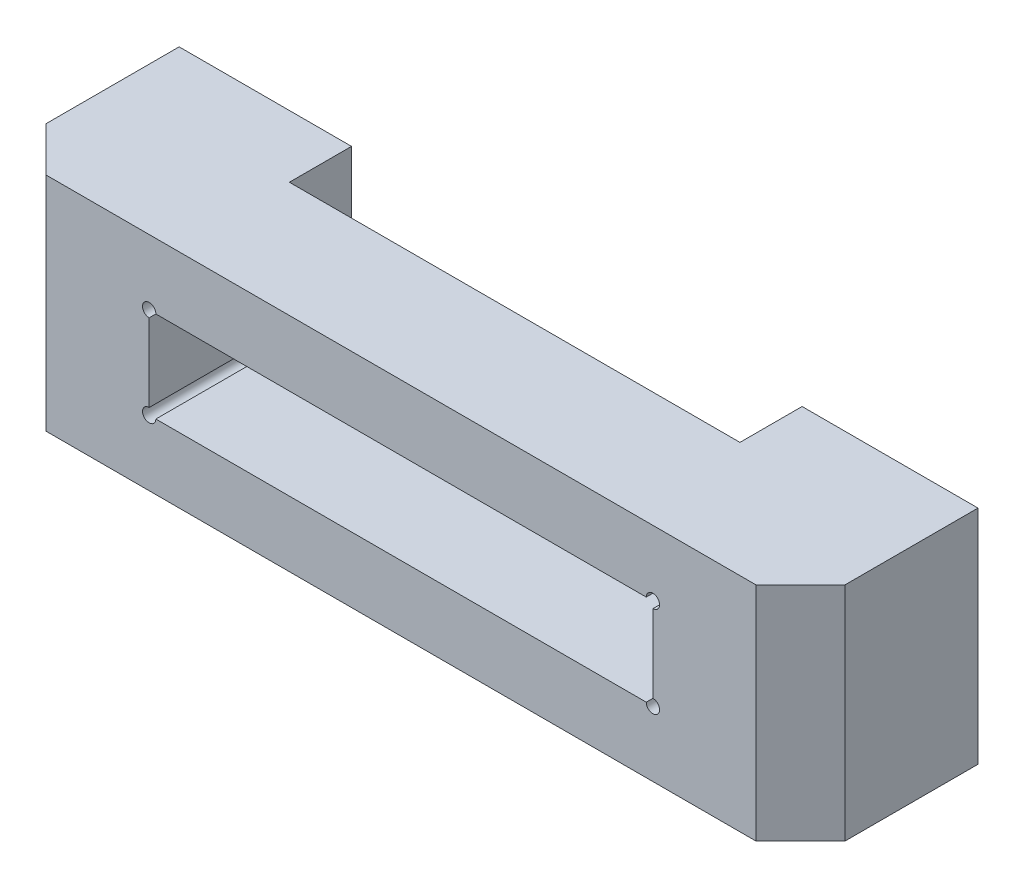
from build123d import *

# Parameters (mm, degrees)
SKETCH1_W           = 180
SKETCH1_H           = 50
BOSS_EXTRUDE1_DEPTH = 40
SKETCH2_W           = 113.5
SKETCH2_H           = 20.5
CUT_EXTRUDE1_DEPTH  = 102.612007165
SKETCH3_R           = 1.5
CUT_EXTRUDE2_DEPTH  = 102.612007165
SKETCH4_W           = 101.523941395
SKETCH4_H           = 14
CUT_EXTRUDE3_DEPTH  = 30
SKETCH5_W           = 113.5
SKETCH5_H           = 14.75
CUT_EXTRUDE4_DEPTH  = 14
CHAMFER1_SIZE       = 10


with BuildPart() as part:
    # Sketch1 → Boss-Extrude1 (new body)
    with BuildSketch(Plane.XY):
        Rectangle(SKETCH1_W, SKETCH1_H)
    extrude(amount=BOSS_EXTRUDE1_DEPTH)

    # Sketch2 → Cut-Extrude1 (cut, through all)
    with BuildSketch(Plane.XY.offset(40)):
        Rectangle(SKETCH2_W, SKETCH2_H)
    extrude(amount=-CUT_EXTRUDE1_DEPTH, mode=Mode.SUBTRACT)

    # Sketch3 → Cut-Extrude2 (cut, through all)
    with BuildSketch(Plane.XY.offset(40)):
        with Locations((-56.75, 10.25)):
            Circle(SKETCH3_R)
        with Locations((-56.75, -10.25)):
            Circle(SKETCH3_R)
        with Locations((56.75, 10.25)):
            Circle(SKETCH3_R)
        with Locations((56.75, -10.25)):
            Circle(SKETCH3_R)
    extrude(amount=-CUT_EXTRUDE2_DEPTH, mode=Mode.SUBTRACT)

    # Sketch4 → Cut-Extrude3 (cut)
    with BuildSketch(Plane(origin=(0, 25, 0), x_dir=(1, 0, 0), z_dir=(0, 1, 0))):
        with Locations((-0.398466407, -7)):
            Rectangle(SKETCH4_W, SKETCH4_H)
    extrude(amount=-CUT_EXTRUDE3_DEPTH, mode=Mode.SUBTRACT)

    # Sketch5 → Cut-Extrude4 (cut)
    with BuildSketch(Plane(origin=(0, 0, 0), x_dir=(-1, 0, 0), z_dir=(0, 0, -1))):
        with Locations((0, -17.625)):
            Rectangle(SKETCH5_W, SKETCH5_H)
    extrude(amount=-CUT_EXTRUDE4_DEPTH, mode=Mode.SUBTRACT)

    # Chamfer1
    chamfer1_edges = [part.edges().sort_by_distance(p)[0] for p in [
        (90, 0, 40),
        (-90, 0, 40),
    ]]
    chamfer(chamfer1_edges, length=CHAMFER1_SIZE)


solid = part.part
